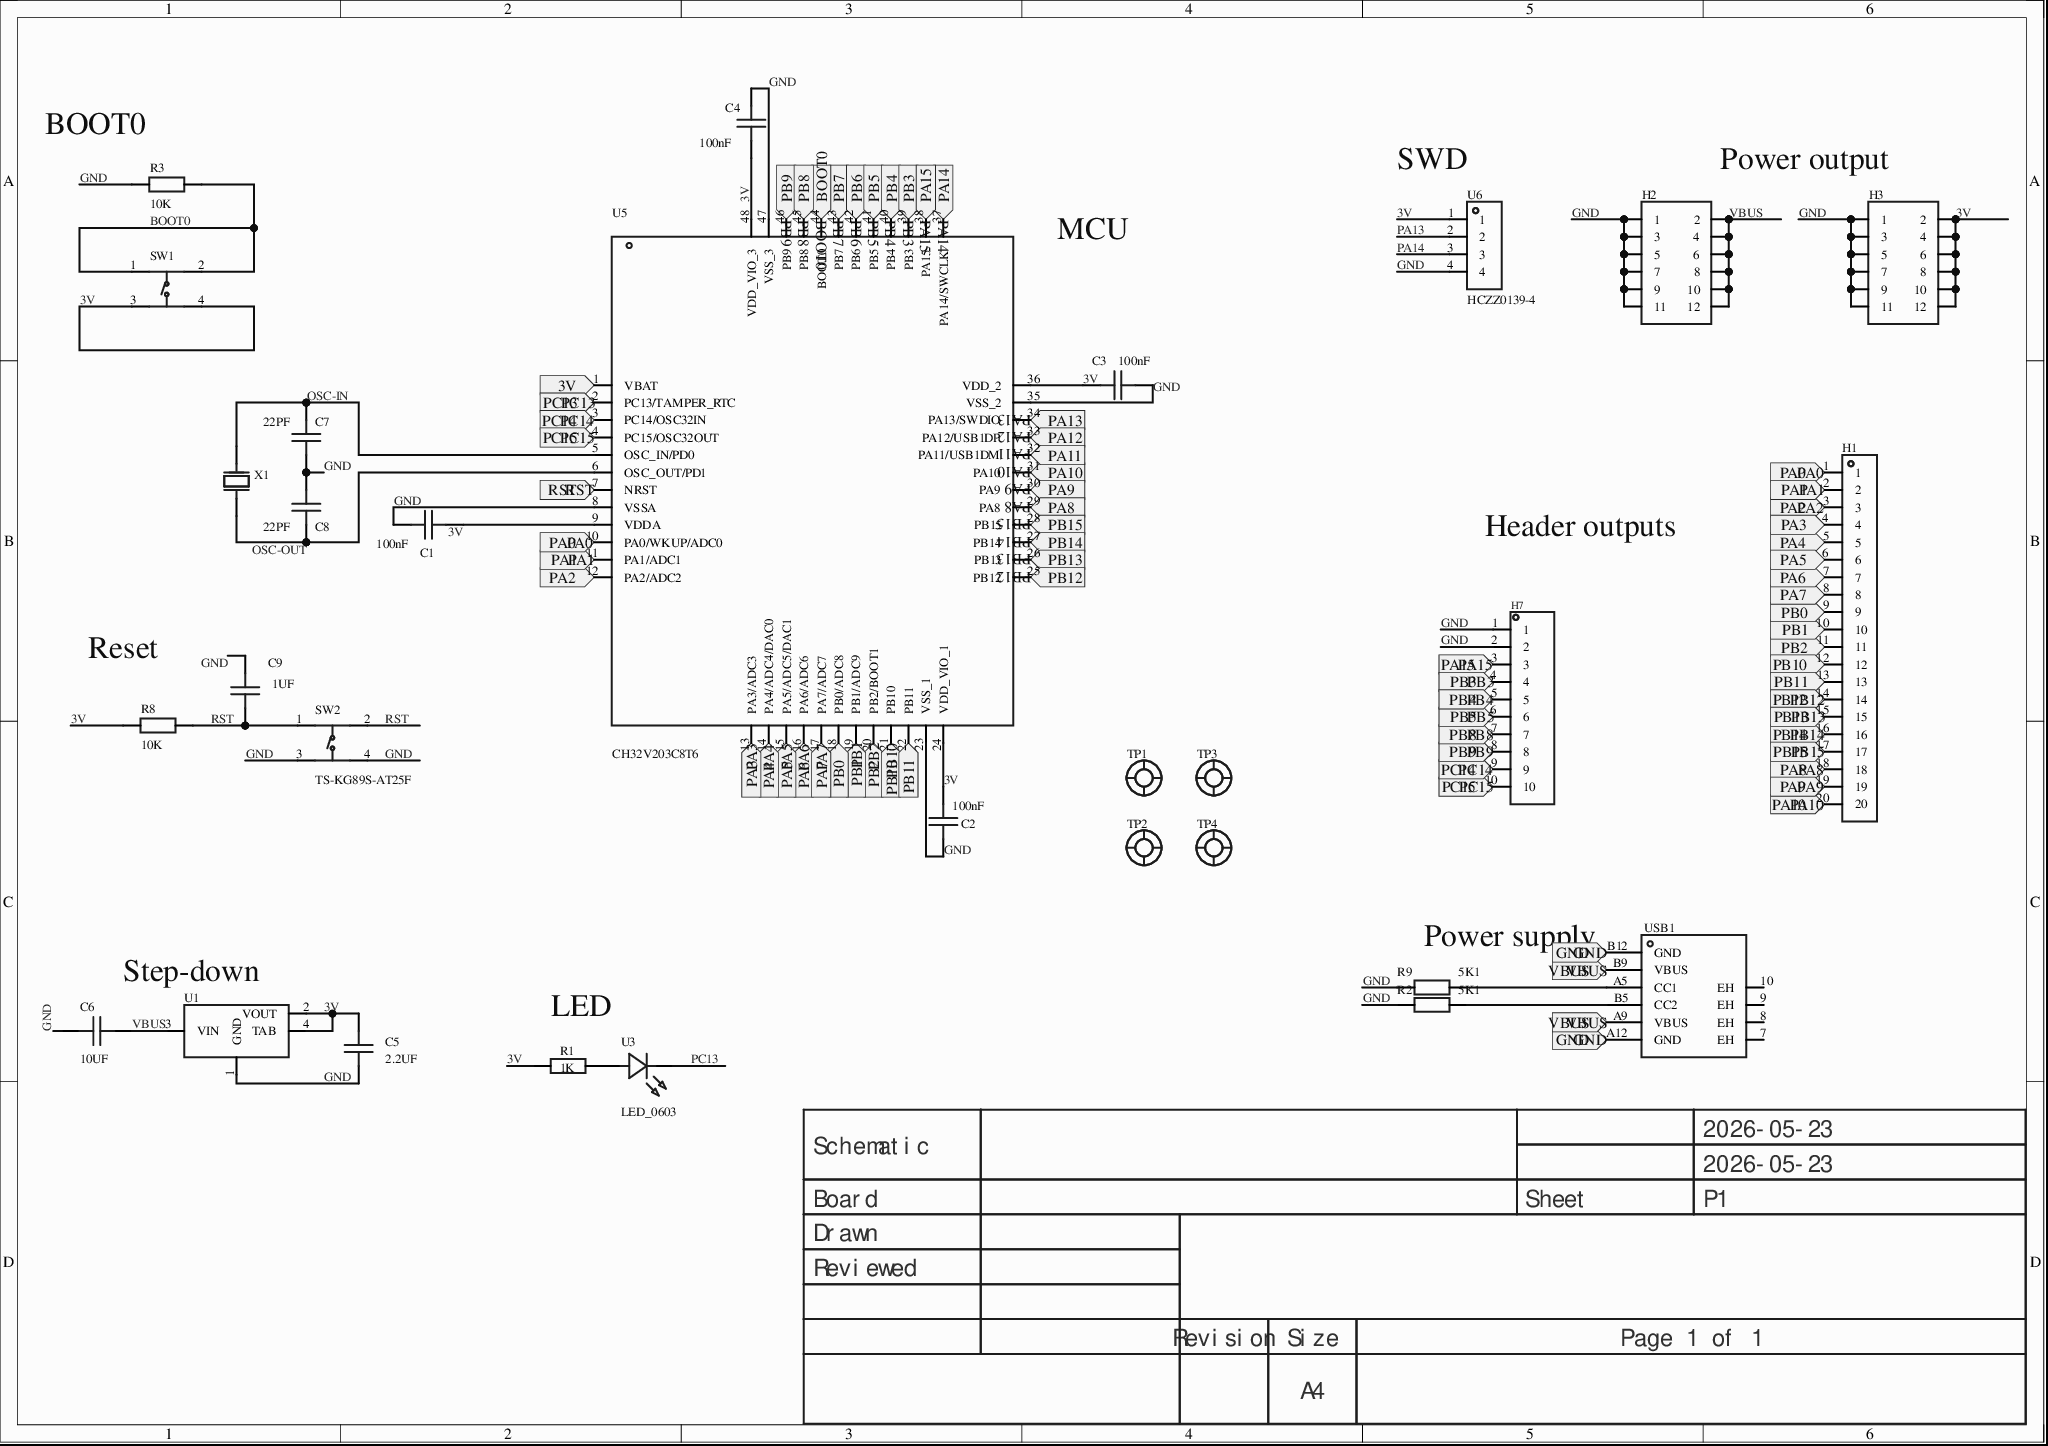
[diagram p0: MISC89146-3.schdoc]
# Altium project MISC89146-2.PrjPcb
1 sheet, 30 parts. Net scope: flat (ports and power ports of the same name join across sheets).
Board file: MISC89146.pcbdoc

## Sheet MISC89146-3.schdoc
size 297 x 209 mm; Version: V1.0; @Project Name: MISC89146; @Update Date: 2026-05-23; @Create Date: 2026-05-23; @Board Name: MISC89146; @Create Time: 10:39:30; @Page Count: 1; @Page No: 1; @Schematic Name: MISC89146; @Update Time: 10:39:30; Size: A4

### Parts
C1  100nF  [C0603]
C2  100nF  [C0603]
C3  100nF  [C0603]
C4  100nF  [C0603]
C5  2.2UF  [C0603]
C6  10UF  [C0603]
C7  22PF  [C0603]
C8  22PF  [C0603]
C9  1UF  [C0603]
H1  (no value)  [HDR-TH_20P-P2.54-V-M-1]
H2  (no value)  [HDR-TH_12P-P2.54-V-M-R2-C6-S2.54]
H3  (no value)  [HDR-TH_12P-P2.54-V-M-R2-C6-S2.54]
H7  (no value)  [hdr-th_10p-p2.54-v-m-1]
R1  1K  [R0603]
R2  5K1  [R0603]
R3  10K  [R0603]
R8  10K  [R0603]
R9  5K1  [R0603]
SW1  TS-KG89S-AT25F  [SW-SMD_4P-L4.2-W3.3-P2.15-LS5.1]  (value not drawn)
SW2  TS-KG89S-AT25F  [SW-SMD_4P-L4.2-W3.3-P2.15-LS5.1]
TP1  (no value)  [M3]
TP2  (no value)  [M3]
TP3  (no value)  [M3]
TP4  (no value)  [M3]
U1  (no value)  [SOT_223]
U3  LED_0603  [LED_0603]
U5  CH32V203C8T6  [LQFP-48_L7.0-W7.0-P0.50-LS9.0-BL]
U6  HCZZ0139-4  [CONN-TH_4P-P2.50_HCZZ0139-4]
USB1  (no value)  [USB_ TYPE-C-6P]
X1  8M-HC-49SMD  [CRYSTAL-SMD_L11.4-W4.7-LS12.7]  (value not drawn)

### Ports
3V (in), BOOT0 (in), GND (in), PA0 (in), PA1 (in), PA2 (in), PA3 (in), PA4 (in), PA5 (in), PA6 (in), PA7 (in), PA8 (in), PA9 (in), PA10 (in), PA11 (in), PA12 (in), PA13 (in), PA14 (in), PA15 (in), PB0 (in), PB1 (in), PB2 (in), PB3 (in), PB4 (in), PB5 (in), PB6 (in), PB7 (in), PB8 (in), PB9 (in), PB10 (in), PB11 (in), PB12 (in), PB13 (in), PB14 (in), PB15 (in), PC13 (in), PC14 (in), PC15 (in), RST (in), VBUS (in)

### Nets
3V: C1.1 C2.2 C3.2 C4.1 C5.1 H3.2 H3.4 H3.6 H3.8 H3.10 H3.12 R1.1 R8.1 SW1.3 SW1.4 U1.2(VOUT) U1.4(TAB) U5.9(VDDA) U5.24(VDD_VIO_1) U5.36(VDD_2) U5.48(VDD_VIO_3) U6.1
BOOT0: R3.2 SW1.1 SW1.2 U5.44(BOOT0) ; port BOOT0
GND: C1.2 C2.1 C3.1 C4.2 C5.2 C6.1 C7.1 C8.2 C9.2 H2.1 H2.3 H2.5 H2.7 H2.9 H2.11 H3.1 H3.3 H3.5 H3.7 H3.9 H3.11 H7.1 H7.2 R2.1 R3.1 R9.1 SW2.3 SW2.4 U1.1(GND) U5.8(VSSA) U5.23(VSS_1) U5.35(VSS_2) U5.47(VSS_3) U6.4 USB1.A12(GND) USB1.B12(GND) ; port GND
OSC-IN: C7.2 U5.5(OSC_IN/PD0) X1.2(OSC2)
OSC-OUT: C8.1 U5.6(OSC_OUT/PD1) X1.1(OSC1)
PA0: H1.1 U5.10(PA0/WKUP/ADC0) ; port PA0
PA1: H1.2 U5.11(PA1/ADC1) ; port PA1
PA2: H1.3 U5.12(PA2/ADC2) ; port PA2
PA3: H1.4 U5.13(PA3/ADC3) ; port PA3
PA4: H1.5 U5.14(PA4/ADC4/DAC0) ; port PA4
PA5: H1.6 U5.15(PA5/ADC5/DAC1) ; port PA5
PA6: H1.7 U5.16(PA6/ADC6) ; port PA6
PA7: H1.8 U5.17(PA7/ADC7) ; port PA7
PA8: H1.18 U5.29(PA8) ; port PA8
PA9: H1.19 U5.30(PA9) ; port PA9
PA10: H1.20 U5.31(PA10) ; port PA10
PA11: U5.32(PA11/USB1DM) ; port PA11
PA12: U5.33(PA12/USB1DP) ; port PA12
PA13: U5.34(PA13/SWDIO) U6.2 ; port PA13
PA14: U5.37(PA14/SWCLK) U6.3 ; port PA14
PA15: H7.3 U5.38(PA15) ; port PA15
PB1: H1.10 U5.19(PB1/ADC9) ; port PB1
PB2: H1.11 U5.20(PB2/BOOT1) ; port PB2
PB3: H7.4 U5.39(PB3) ; port PB3
PB4: H7.5 U5.40(PB4) ; port PB4
PB5: H7.6 U5.41(PB5) ; port PB5
PB6: U5.42(PB6) ; port PB6
PB7: U5.43(PB7) ; port PB7
PB8: H7.7 U5.45(PB8) ; port PB8
PB9: H7.8 U5.46(PB9) ; port PB9
PB10: H1.12 U5.21(PB10) ; port PB10
PB12: H1.14 U5.25(PB12) ; port PB12
PB13: H1.15 U5.26(PB13) ; port PB13
PB14: H1.16 U5.27(PB14) ; port PB14
PB15: H1.17 U5.28(PB15) ; port PB15
PC13: U3.1(K) U5.2(PC13/TAMPER_RTC) ; port PC13
PC14: H7.9 U5.3(PC14/OSC32IN) ; port PC14
PC15: H7.10 U5.4(PC15/OSC32OUT) ; port PC15
RST: C9.1 R8.2 SW2.1 SW2.2 U5.7(NRST) ; port RST
VBUS: C6.2 H2.2 H2.4 H2.6 H2.8 H2.10 H2.12 U1.3(VIN) USB1.A9(VBUS) USB1.B9(VBUS) ; port VBUS
NetH1_9: H1.9 U5.18(PB0/ADC8) ; port PB0
NetH1_13: H1.13 U5.22(PB11) ; port PB11
NetR1_2: R1.2 U3.2(A)
NetR2_2: R2.2 USB1.B5(CC2)
NetR9_2: R9.2 USB1.A5(CC1)
NetU5_1: U5.1(VBAT) ; port 3V

Not connected (* = marked no-connect by the designer): TP1 0*; TP2 0*; TP3 0*; TP4 0*; USB1 7(EH) 8(EH) 9(EH) 10(EH)

### Notes on the sheet
- (near R3) BOOT0
- (near U6) SWD
- Power output
- (near U5) MCU
- Header outputs
- Reset
- Power supply
- Step-down
- LED
- 2026-05-23
- Schematic
- Board
- Sheet
- P1
- Drawn
- Reviewed
- Revision
- Size
- A4
- Page 1 of 1

### Library data of the parts
C1-C9 = CAP_0603: Symbol: C1210X7R475K630NT; 3D Model: ac125912035d415993ca9572d50418b1; 3D Model Transform: 62.992,31.496,0,0,0,0,0,0,0; ConvertToPcb: yes; ModelName: C0603_L1.6-W0.8-H0.8; Device: CAP_0603; Supplier: LCSC; Supplier Footprint: 0603; AddInBom: yes; FootprintName: C0603
  C1-C4: Value: 100nF; Supplier Part: C14663
  C5: Value: 2.2UF
  C6: Value: 10UF; Supplier Part: C326057
  C7 C8: Value: 22PF; Supplier Part: C91701
  C9: Value: 1UF; Supplier Part: C106214
H1 = HDR-M_2.54_1x20P: Pitch:2.54mm;Total pins:20;Rows:1;Pin structure:-;Row spacing:-;Mounting type:Through-hole;Round/square pin:-;Rated current:-;Rated voltage:-;Mating pin length:-;Plastic height:-;Contact material:Brass;Contact plating:-;Color:Black;; 3D Model: f68709be121d406db68b06f32a595389; 3D Model Transform: 1999.996,100,0,0,0,0,0,2.48,-118.11; ConvertToPcb: yes; ModelName: HDR-M-2.54_1x20; Symbol: HDR-M_2.54_1x20P; Device: HDR-M_2.54_1x20P; Supplier Part: C50981; Supplier Footprint: 插件; AddInBom: yes; FootprintName: HDR-TH_20P-P2.54-V-M-1
H2 H3 = HDR-F_2.54_2x6: Symbol: HDR-F-2.54_2x6; AddInBom: yes; ModelId: 390ea0804e1641cbaab12298c8a540710819f05c4eef4c71ace90d822a990e87; ModelName: HDR2.54-M-LI-2X6P; ModelTransform: 599.999,200,0,0,0,0,0,0,-118.11; Device: HDR-F_2.54_2x6; ConvertToPcb: yes; FootprintName: HDR-TH_12P-P2.54-V-M-R2-C6-S2.54
H7 = HDR-M_2.54_1x10P: Manufacturer Part: 2.54-1*10P针; Manufacturer: BOOMELE(博穆精密); Symbol: Header-Male-2.54_1x10; 3D Model: 10f3d1cea59e4bb4ba116af9f09c2b9b; 3D Model Transform: 999.99796,100,0,0,0,0,0,0,-118.11; ConvertToPcb: yes; ModelName: HDR2.54-M-LI-1X10P; Device: HDR-M_2.54_1x10P; Supplier Footprint: 插件; Supplier: LCSC; Supplier Part: C57369; JLCPCB Part Class: Extended Part; AddInBom: yes; FootprintName: hdr-th_10p-p2.54-v-m-1
R1-R3 R8 R9 = Res_0603: Symbol: Resistor; 3D Model: 8176a32bb9f4431db75ab5f6460c2416; 3D Model Transform: 63,31.5,20.1,0,0,0,0,0,0; ConvertToPcb: yes; ModelName: R0603_L1.6-W0.8-H0.5; Device: Res_0603; Supplier: LCSC; Supplier Footprint: 0603; AddInBom: yes; FootprintName: R0603
  R1: Value: 1K; Supplier Part: C2907113
  R2 R9: Value: 5K1; Supplier Part: C2907114
  R3 R8: Value: 10K; Supplier Part: C2930027
SW1 SW2 = 4.2*3.25*2.5mm-立贴-轻触开关: Contact current:50mA;Rated voltage (DC):12V;Insulation resistance:100MΩ;Circuit:SPST;Mounting:Vertical SMD;Actuating force:250gf@±50gf;Mechanical life:10万 cycles;With bracket:No;; Manufacturer: HANBO(汉博); Symbol: 4.2*3.25*2.5mm-vertical SMD-tact switch; Contact Current: 50mA; Voltage Rating (DC): 12V; Insulation Resistance: 100MΩ; Circuit: SPST; Actuator Style: Oval button; Actuator/Cap Color: White; Pin Style: SMD tab; Switch Length: 4.2mm; Switch Width: 3.25mm; Switch Height: 2.5mm; Strike Gundam: No; 3D Model: 101da67941e24d4e9615179a94fc6132; 3D Model Transform: 204.724,127.9525,0,0,0,0,0,0,0; AddInBom: yes; ModelName: SW-SMD_4P-L4.2-W3.3-H2.5-P2.15-LS5.1; Device: 4.2*3.25*2.5mm-vertical SMD-tact switch; LCSC Part Name: 4.2*3.25*2.5mm 立贴 轻触开关; Supplier Part: C318904; Manufacturer Part: TS-KG89S-AT25F; Supplier Footprint: SMD; Datasheet: example.com/upload/public/pdf/source/20221110/0D75E68DCC1CEC2670E8A2B9A9134A65.pdf; Supplier: LCSC; Mounting Style: Vertical SMD; Operating Force: 250gf@±50gf; Mechanical Life: 10万 cycles; ConvertToPcb: yes; FootprintName: SW-SMD_4P-L4.2-W3.3-P2.15-LS5.1
TP1-TP4 = M3: Manufacturer: Shuntian(顺天五金); Manufacturer Part: M3x10+6; AddInBom: yes; Symbol: M3; Device: M3; Supplier: LCSC; Supplier Part: C551322; JLCPCB Part Class: Extended library; ConvertToPcb: yes; FootprintName: M3
U1 = AMS1117: Symbol: AMS1117_OLD; AddInBom: yes; ModelId: 925194bf9823436183a3e0b978a8d0760819f05c4eef4c71ace90d822a990e87; ModelName: SOT-223-4P_L6.5-W3.5-H1.6-LS7.0-P2.30; ModelTransform: 279.84,255.85,68.86,90,0,0,0,0,0; Device: AMS1117; ConvertToPcb: yes; FootprintName: SOT_223
U3 = LED_0603_W: 3D Model: 74041d3a270d435c8600a9ab9b7641c0; 3D Model Transform: 63.7794,31.496,0,0,0,0,0,0,0; AddInBom: yes; ModelName: LED0603-RD_RED; Symbol: LED_0603_W; Device: LED_0603_W; LCSC Part Name: LED_0603; Supplier Part: C83904; Manufacturer Part: LED_0603; Supplier Footprint: LEDRED; Supplier: LCSC; ConvertToPcb: yes; FootprintName: LED_0603
U5 = CH32V203C8T6: CPU core:RISC-V;Program storage capacity:64KB;Total RAM:20KB;GPIO port count:-;Operating voltage range:-;Max CPU frequency:144MHz;Program memory type:FLASH;; Manufacturer: WCH(南京沁恒); AddInBom: yes; ModelId: 093be70396ff421eb2cdb946d5311efc0819f05c4eef4c71ace90d822a990e87; ModelName: LQFP-48_L7.0-W7.0-H1.4-LS9.0-P0.50; ModelTransform: 354.331,354.331,0,0,0,0,0,0,0; CPU Core: RISC-V; Program Storage Size: 64KB; RAM Size: 20KB; CPU Maximum Speed: 144MHz; Program Memory Type: FLASH; Symbol: CH32V203C8T6; Device: CH32V203C8T6; LCSC Part Name: CH32V203C8T6; SupplierPart: C3001172; ManufacturerPart: CH32V203C8T6; Supplier Footprint: LQFP-48(7x7); JLCPCB Part Class: Extended Part; Datasheet: example.com/upload/public/pdf/source/20220425/D3E728E801B9982E2758AC225E3A30F9.pdf; Supplier: LCSC; ConvertToPcb: yes; FootprintName: LQFP-48_L7.0-W7.0-P0.50-LS9.0-BL; GPIO Ports Number: -; Operating Voltage Range: -; Operating Temperature Range: -; ADC (Bit): -; DAC (Bit): -; PWM (Bit): -; 8Bit Timer: -; 16Bit Timer: -; 32Bit Timer: -; CAN: -; UART/USART: -; I2C: -; I2S: -; SPI: -; Universal Serial Bus: -; Internal Comparator: -; Peripheral/Function: -; communication protocol: -; Watchdog: -; Real-Time Clock: -; Infrared Data Association: -; Low-Voltage Detect: -; CCP Capture/Compare: -; Secure Digital Input and Output: -; Direct Memory Access: -; Internal Oscillator: -
U6 = XH2.54_弯针_x4P: Pin structure:1x4P;Pitch:2.54mm;Mounting:Right-angle THT;Reference series:XH;Total pins:4P;Rows:1;Pins per row:4;Rated current:3A;Contact material:Brass;Contact plating:Tin;Operating temperature range:-25℃~+85℃;; Manufacturer: HC(虹成电子); Symbol: XH2.54_bent-pin_x4P; 3D Model: 18f8f032edff42ae85e7fd7f8dbffc48; 3D Model Transform: 492.5187,302.16475,0,0,0,0,-0.002,-138.779,-133.858; Pins Structure: 1x4P; Pitch: 2.54mm; Reference Series: XH; Number of PINs Per Row: 4; Current Rating (Max): 3A; AddInBom: yes; Device: XH2.54_bent-pin_x4P; LCSC Part Name: 1x4P 间距:2.54mm 弯插 系列:XH 米色; Supplier Part: C7433739; Manufacturer Part: HCZZ0139-4; Supplier Footprint: 弯插,p=2.54mm; Datasheet: example.com/upload/public/pdf/source/20230707/FBA9049739106B85D22D534C829006CC.pdf; Supplier: LCSC; Mounting Style: Right-angle THT; Number of Pins: 4P; Number of Rows: 1; Contact Material: Brass; Contact Plating: Tin; Operating Temperature Range: -25℃~+85℃; ConvertToPcb: yes; FootprintName: CONN-TH_4P-P2.50_HCZZ0139-4; ModelName: CONN-TH_4P-P2.50_HCZZ0139-4
USB1 = USB_ Type-C-6P: AddInBom: yes; ModelId: d4f492a4e6024845a13b3f6a4ef2d2cb0819f05c4eef4c71ace90d822a990e87; ModelName: USB-SMD_U262-061N-4BVC11; ModelTransform: 352.362,281.496,0,0,0,0,0,-47.244,-39.37; Symbol: USB_ TYPE-C-6P; Device: USB_ Type-C-6P; Supplier Footprint: SMD; ConvertToPcb: yes; FootprintName: USB_ TYPE-C-6P
X1 = HC-49SMD: 3D Model: be19d32e6d024fb4863eb8f4e3f5efcc; 3D Model Transform: 499.999,185.039,0,0,0,0,0,0,0; AddInBom: yes; Symbol: HC-49SMD; Device: HC-49SMD; Supplier Part: C2842263; LCSC Part Name: 8M-HC-49SMD; Manufacturer Part: 8M-HC-49SMD; Supplier Footprint: HC-49SMD; JLCPCB Part Class: Extended library; Supplier: LCSC; ConvertToPcb: yes; FootprintName: CRYSTAL-SMD_L11.4-W4.7-LS12.7; ModelName: CRYSTAL-SMD_L11.4-W4.7-LS12.7